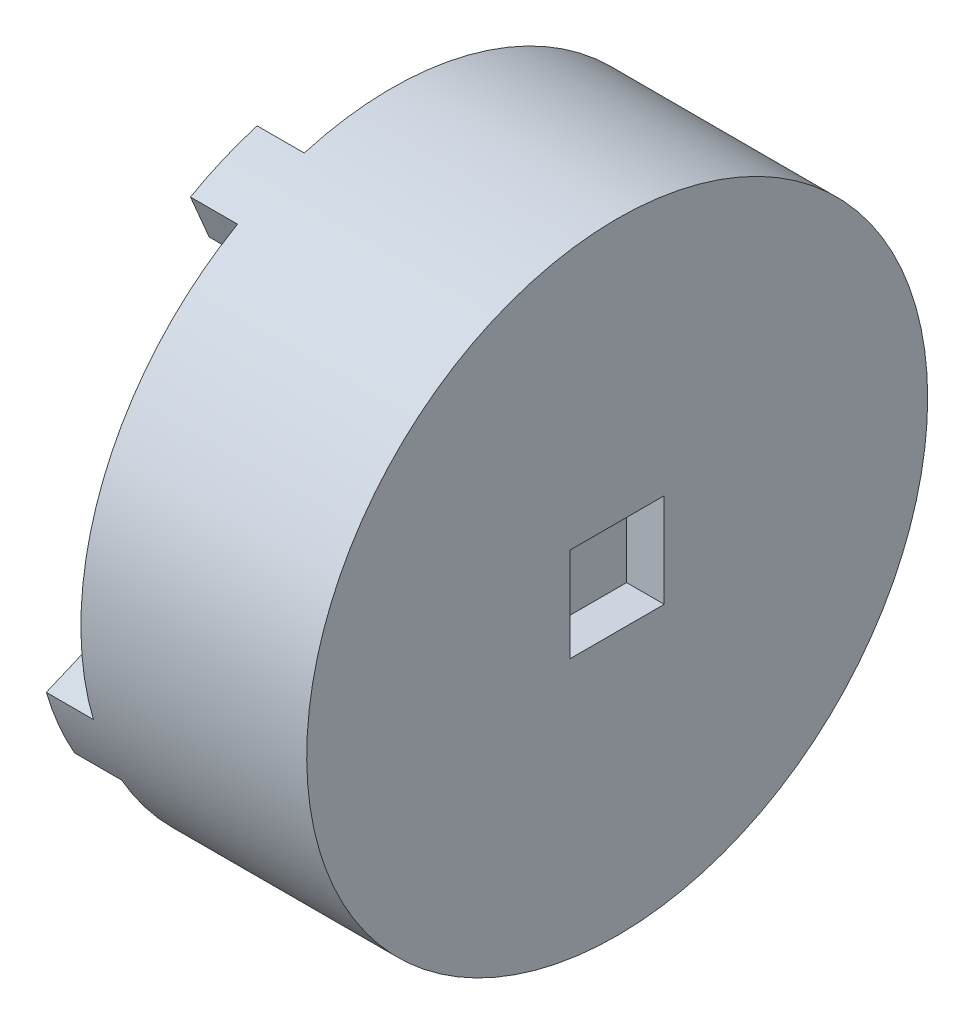
SolidWorks part; units mm, degrees
material "电木（PF）"
ref_plane "前视基准面" through (0, 0, 0) normal (0, 0, 1) x (1, 0, 0)
ref_plane "上视基准面" through (0, 0, 0) normal (0, 1, 0) x (1, 0, 0)
ref_plane "右视基准面" through (0, 0, 0) normal (1, 0, 0) x (0, 0, -1)
sketch "草图1" plane through (0, 0, 0) normal (1, 0, 0) x (0, 0, -1)
  circle A0 centre (0, 0) radius 16.5
  dimension "D1" = 33
extrude "凸台-拉伸1" add sketch "草图1" along normal blind 12
sketch "草图2" plane through (0, 0, 0) normal (-1, 0, 0) x (0, 0, 1)
  circle A0 centre (0, 0) radius 3.75
  dimension "D1" = 7.5
extrude "切除-拉伸1" cut sketch "草图2" against normal blind 4
sketch "草图3" plane through (0, 0, 0) normal (-1, 0, 0) x (0, 0, 1)
  line L0 (-3.6397, -13.5011) -> (-4.6311, -15.8368)
  line L1 (-3.4443, -13.0409) -> (-4.6311, -15.8368) construction
  line L2 (-3.6397, -13.5011) -> (-7.1836, -11.9968)
  line L3 (-8.175, -14.3325) -> (-6.9882, -11.5366) construction
  line L4 (-7.1836, -11.9968) -> (-8.175, -14.3325)
  line L5 (-6.9882, -11.5366) -> (-3.4443, -13.0409) construction
  circle A0 centre (0, 0) radius 16.5 construction
  arc A1 (-8.175, -14.3325) -> (-4.6311, -15.8368) centre (0, 0) ccw
  dimension "D1" = 0.5
extrude "凸台-拉伸2" add sketch "草图3" along normal blind 2.5
pattern_circular "阵列(圆周)1" count 4 over 360 about axis through (0, 0, 0) along (1, 0, 0) of "凸台-拉伸2"
sketch "草图4" plane through (0, 0, 0) normal (-1, 0, 0) x (0, 0, 1)
  line L0 (-1.6496, 11.3838) -> (-0.9157, 9.5093) construction
  line L1 (0.9157, -9.5093) -> (1.6496, -11.3838) construction
  circle A0 centre (-1.2827, 10.4465) radius 2.25
  circle A1 centre (1.2827, -10.4465) radius 2
  dimension "D1" = 4.5
  dimension "D2" = 4
extrude "切除-拉伸2" cut sketch "草图4" against normal up to surface (4 mm away) up to face at (4, 0, 3.75)
sketch "草图5" plane through (12, 0, 0) normal (1, 0, 0) x (0, 0, -1)
  line L1 (-2.5, 2.5) -> (2.5, 2.5)
  line L2 (-2.5, 2.5) -> (-2.5, -2.5)
  line L3 (-2.5, -2.5) -> (2.5, -2.5)
  line L4 (2.5, 2.5) -> (2.5, -2.5)
  line L5 (-2.5, 2.5) -> (2.5, -2.5) construction
  line L6 (-2.5, -2.5) -> (2.5, 2.5) construction
  point P0 (0, 0)
  dimension "D1" = 5
  dimension "D2" = 5
extrude "切除-拉伸3" cut sketch "草图5" against normal blind 2
